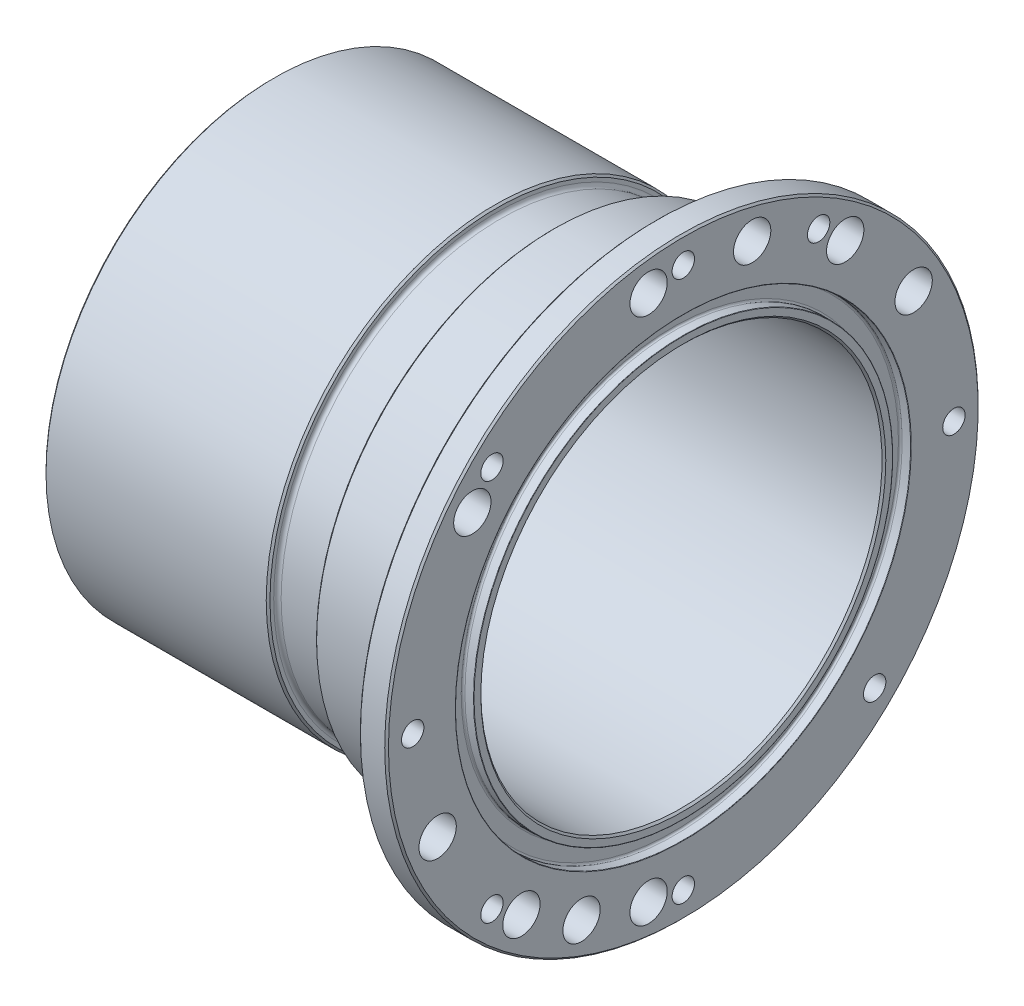
SolidWorks part; units mm, degrees
material "42CrMo"
ref_plane "Front Plane" through (0, 0, 0) normal (0, 0, 1) x (1, 0, 0)
ref_plane "Top Plane" through (0, 0, 0) normal (0, 1, 0) x (1, 0, 0)
ref_plane "Right Plane" through (0, 0, 0) normal (1, 0, 0) x (0, 0, -1)
sketch "Sketch1" plane through (0, 0, 0) normal (0, 0, 1) x (1, 0, 0)
  line L0 (0, 0) -> (199.4668, 0) construction
  line L1 (0, 0) -> (0, 180.6572) construction
  line L2 (0, 107.5) -> (220, 107.5)
  line L3 (220, 107.5) -> (220, 112.1)
  line L4 (219.8, 112.3) -> (215.28, 112.3)
  line L5 (214.28, 113.3) -> (214.28, 121)
  line L6 (215.28, 122) -> (219.8, 122)
  line L7 (220, 122.2) -> (220, 159)
  line L8 (220, 159) -> (205, 159)
  line L9 (205, 159) -> (205, 127.5)
  line L10 (205, 127.5) -> (150, 127.5)
  line L11 (150, 127.5) -> (150, 117.5)
  line L12 (150, 117.5) -> (120, 117.5)
  line L13 (120, 117.5) -> (120, 122.5)
  line L14 (120, 122.5) -> (0, 122.5)
  line L15 (0, 122.5) -> (0, 107.5)
  arc A0 (214.28, 121) -> (215.28, 122) centre (215.28, 121) cw
  arc A1 (215.28, 112.3) -> (214.28, 113.3) centre (215.28, 113.3) cw
  arc A2 (220, 112.1) -> (219.8, 112.3) centre (219.8, 112.1) ccw
  arc A3 (219.8, 122) -> (220, 122.2) centre (219.8, 122.2) ccw
  dimension "D12" = 1
  dimension "D13" = 0.2
  dimension "D1" = 107.5
  dimension "D2" = 10
  dimension "D3" = 15
  dimension "D4" = 15
  dimension "D5" = 220
  dimension "D6" = 30
  dimension "D7" = 120
  dimension "D8" = 20
  dimension "D9" = 159
  dimension "D10" = 5.72
  dimension "D11" = 9.7
  dimension "D14" = 122
revolve "Revolve1" add sketch "Sketch1" angle 360 about L0
sketch "Sketch2" plane through (205, 0, 0) normal (-1, 0, 0) x (0, 0, 1)
  line L0 (0, 0) -> (145, 0) construction
  line L1 (0, 0) -> (0, 145) construction
  line L2 (0, 0) -> (-72.5, 125.5737) construction
  circle A0 centre (0, 0) radius 145 construction
  circle A1 centre (-72.5, 125.5737) radius 6
  circle A2 centre (0, 145) radius 6
  circle A3 centre (102.5305, 102.5305) radius 6
  circle A4 centre (145, 0) radius 6
  circle A5 centre (102.5305, -102.5305) radius 6
  circle A6 centre (0, -145) radius 6
  circle A7 centre (-102.5305, -102.5305) radius 6
  circle A8 centre (-145, 0) radius 6
  circle A10 centre (-102.5305, 102.5305) radius 6 [skipped]
  point P25 (0, 0)
  dimension "D1" = 290
  dimension "D3" = 12
  dimension "D4" = 12
  dimension "D2" = 30
  dimension "D5" = 8
extrude "Cut-Extrude1" cut sketch "Sketch2" against normal through all
fillet "Fillet1" radius 2 2 edges at (150, 0, 117.5) (120, 0, 117.5)
chamfer "Chamfer1" distance 1 angle 45 6 edges at (220, 0, 159) (205, 0, 159) (120, 0, 122.5) (150, 0, 127.5) (0, 0, 107.5) (0, 0, 122.5)
fillet "Fillet2" radius 2 1 edges at (205, 0, 127.5)
chamfer "Chamfer2" distance 1 angle 45 1 edges at (220, 0, 107.5)
sketch "Sketch3" plane through (0, 0, 0) normal (1, 0, 0) x (0, 0, -1)
  line L0 (0, 0) -> (0, 167.7375) construction
sketch "Sketch4" plane through (205, 0, 0) normal (-1, 0, 0) x (0, 0, 1)
  line L0 (0, 0) -> (18.6, 141.2809) construction
  line L1 (0, 0) -> (-36.8817, 137.6444) construction
  line L2 (0, 0) -> (-86.7485, 113.0529) construction
  line L3 (0, 0) -> (-123.4086, 71.25) construction
  line L4 (0, 0) -> (113.0529, 86.7485) construction
  line L5 (0, 0) -> (158, 0) construction
  line L6 (0, 0) -> (131.6528, -54.5324) construction
  line L7 (0, 0) -> (86.7485, -113.0529) construction
  line L8 (0, 0) -> (54.5324, -131.6528) construction
  line L9 (0, 0) -> (18.6, -141.2809) construction
  line L10 (0, 0) -> (0, 167.7375) construction
  circle A0 centre (0, 0) radius 142.5 construction
  circle A1 centre (0, 0) radius 158 construction
  circle A2 centre (-123.4086, 71.25) radius 10
  circle A3 centre (-86.7485, 113.0529) radius 10
  circle A4 centre (-36.8817, 137.6444) radius 10
  circle A5 centre (18.6, 141.2809) radius 10
  circle A6 centre (113.0529, 86.7485) radius 10
  circle A7 centre (131.6528, -54.5324) radius 10
  circle A8 centre (86.7485, -113.0529) radius 10
  circle A9 centre (54.5324, -131.6528) radius 10
  circle A10 centre (18.6, -141.2809) radius 10
  dimension "D1" = 285
  dimension "D11" = 20
  dimension "D2" = 7.5
  dimension "D3" = 22.5
  dimension "D4" = 22.5
  dimension "D5" = 22.5
  dimension "D6" = 45
  dimension "D7" = 22.5
  dimension "D8" = 30
  dimension "D9" = 15
  dimension "D10" = 15
extrude "Cut-Extrude2" cut sketch "Sketch4" against normal through all
